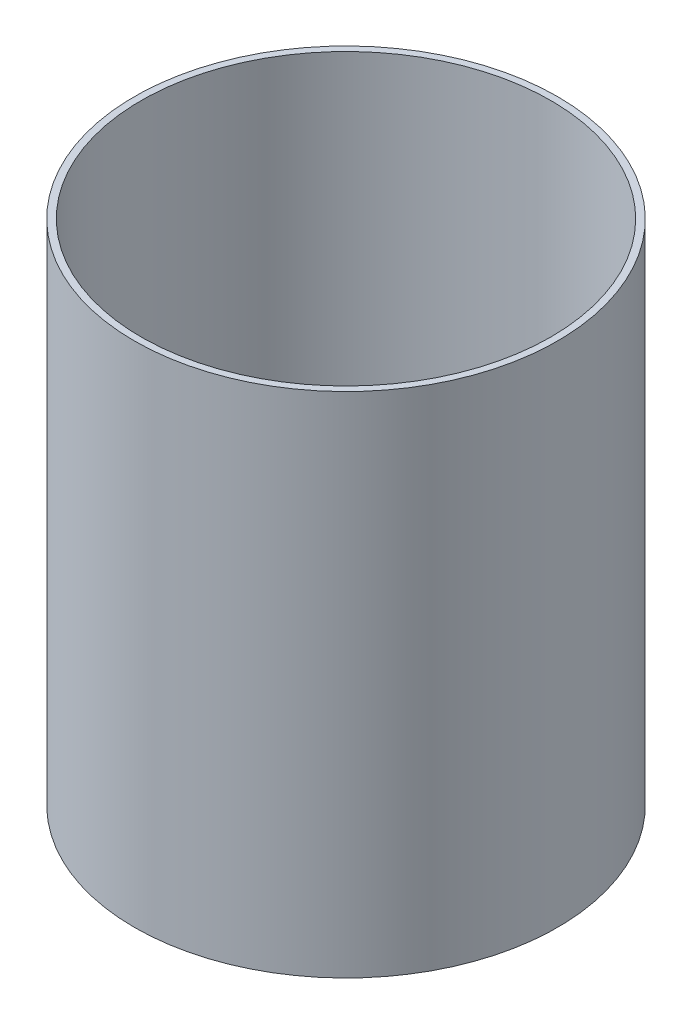
from build123d import *

# Parameters (mm, degrees)
SKETCH_1_R      = 125
SKETCH_1_R_2    = 121
EXTRUDE_1_DEPTH = 300


with BuildPart() as part:
    # 草图1 → 拉伸-薄壁1 (new body)
    with BuildSketch(Plane(origin=(0, 0, 0), x_dir=(1, 0, 0), z_dir=(0, 1, 0))):
        Circle(SKETCH_1_R)
        Circle(SKETCH_1_R_2, mode=Mode.SUBTRACT)
    extrude(amount=EXTRUDE_1_DEPTH)


solid = part.part
